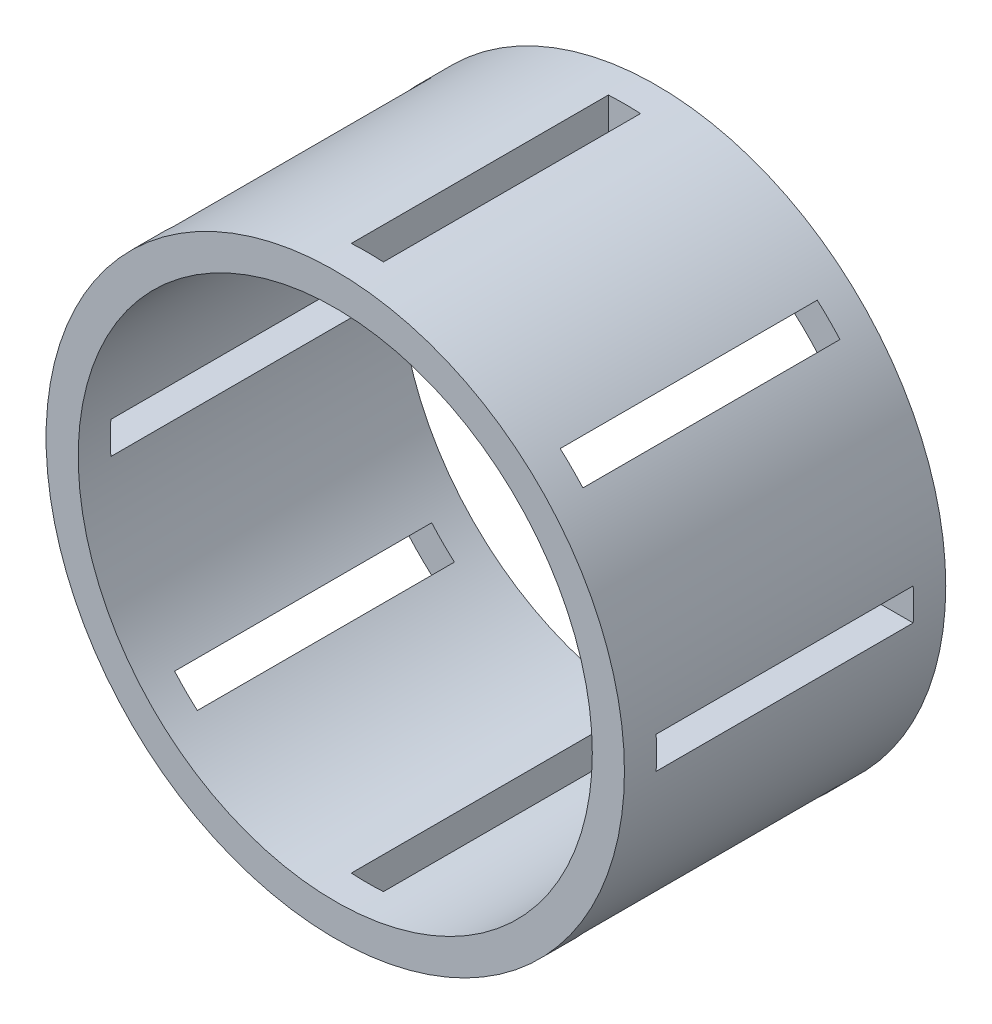
from build123d import *

# Parameters (mm, degrees)
SKETCH1_R           = 45
SKETCH1_R_2         = 40
BOSS_EXTRUDE1_DEPTH = 50
SKETCH2_W           = 5
SKETCH2_H           = 40
CUT_EXTRUDE1_DEPTH  = 661.757616096
CIRPATTERN1_COUNT   = 8


with BuildPart() as part:
    # Sketch1 → Boss-Extrude1 (new body)
    with BuildSketch(Plane.XY):
        with Locations((-599.884196758, -90)):
            Circle(SKETCH1_R)
        with Locations((-599.884196758, -90)):
            Circle(SKETCH1_R_2, mode=Mode.SUBTRACT)
    extrude(amount=BOSS_EXTRUDE1_DEPTH)

    # Sketch2 → Cut-Extrude1 (cut, symmetric)
    with BuildSketch(Plane(origin=(0, 0, 0), x_dir=(1, 0, 0), z_dir=(0, 1, 0))):
        with Locations((-599.884196758, -25)):
            Rectangle(SKETCH2_W, SKETCH2_H)
    cut_extrude1 = extrude(amount=CUT_EXTRUDE1_DEPTH, both=True, mode=Mode.SUBTRACT)

    # CirPattern1: Cut-Extrude1 ×8 about axis
    cirpattern1_axis = Axis((-599.884196758, -90, 0), (0, 0, 1))
    for i in range(1, CIRPATTERN1_COUNT):
        add(cut_extrude1.rotate(cirpattern1_axis, i * 360 / CIRPATTERN1_COUNT), mode=Mode.SUBTRACT)


solid = part.part
